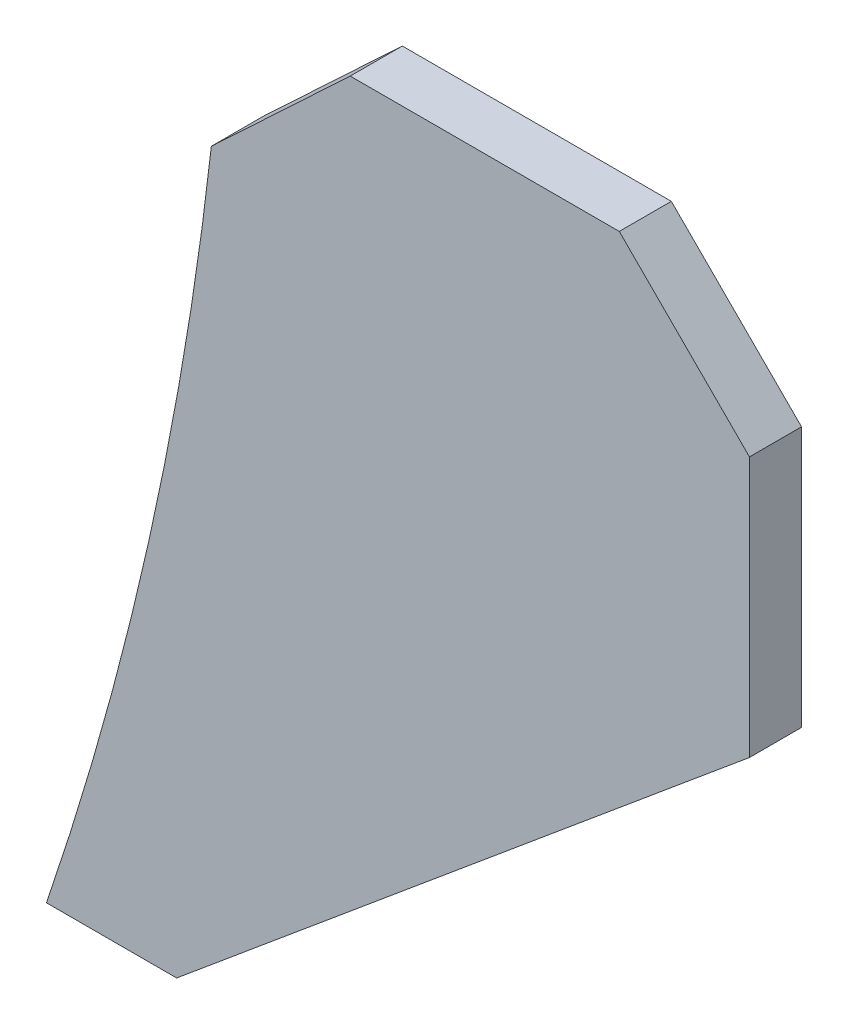
SolidWorks part; units mm, degrees
material "Q235B"
ref_plane "Front Plane" through (0, 0, 0) normal (0, 0, 1) x (1, 0, 0)
ref_plane "Top Plane" through (0, 0, 0) normal (0, 1, 0) x (1, 0, 0)
ref_plane "Right Plane" through (0, 0, 0) normal (1, 0, 0) x (0, 0, -1)
sketch "Sketch1" plane through (0, 0, 0) normal (0, 0, 1) x (1, 0, 0)
  line L0 (0, 0) -> (15, 0)
  line L1 (15, 0) -> (81, 55)
  line L2 (81, 55) -> (81, 85)
  line L3 (81, 85) -> (66, 100)
  line L4 (66, 100) -> (35, 100)
  line L5 (35, 100) -> (19, 85)
  arc A0 (19, 85) -> (0, 0) centre (-383.4544, 130.3369) cw
  dimension "D1" = 405
  dimension "D2" = 15
  dimension "D3" = 30
  dimension "D4" = 45
  dimension "D5" = 31
  dimension "D6" = 46
  dimension "D7" = 62
  dimension "D8" = 81
  dimension "D9" = 100
extrude "Boss-Extrude1" add sketch "Sketch1" along normal blind 6
